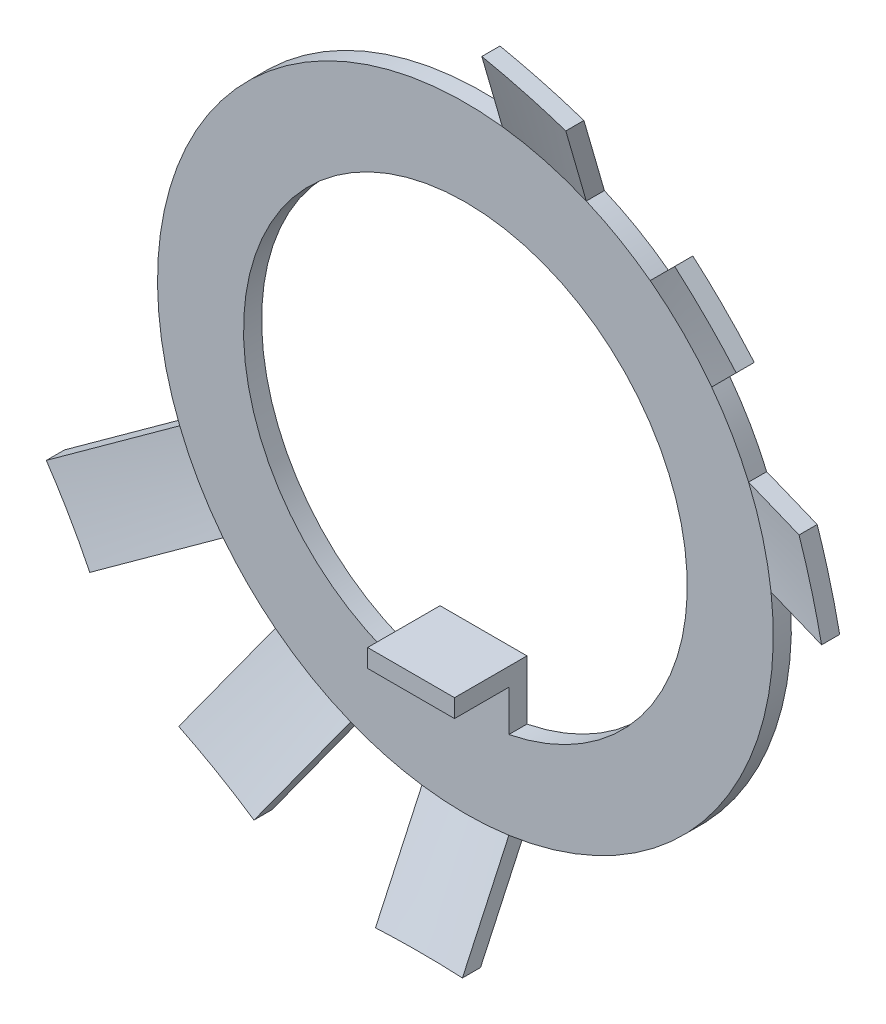
from build123d import *

# Parameters (mm, degrees)
CUT_EXTRUDE2_START  = -3e-06
SKETCH3_OUTSIDE_W   = 59.748
SKETCH3_OUTSIDE_H   = 59.748
CUT_EXTRUDE2_DEPTH  = 3.564697
SKETCH4_W           = 4.8
SKETCH4_H           = 1
BOSS_EXTRUDE1_DEPTH = 4


with BuildPart() as part:
    # Sketch2 → Boss-Revolve (revolve)
    with BuildSketch(Plane(origin=(0, 0, 0), x_dir=(0, 0, -1), z_dir=(1, 0, 0))):
        Polygon((-2.56469212, 22.5), (0, 17), (0, 0), (-1, 0), (-1, 17), (-3.56469212, 22.5), align=None)
    revolve(axis=Axis((0, 0, 0), (0, 0, 1)))

    # Sketch3 outside → Cut-Extrude2 (cut)
    # profile 1 of 2: a face of its own
    with BuildSketch(Plane.XY.offset(CUT_EXTRUDE2_START)):
        Rectangle(SKETCH3_OUTSIDE_W, SKETCH3_OUTSIDE_H)
        with BuildLine():
            Line((-2.4, -16.829735589), (-2.4, -22.371633825))
            Line((-2.4, -22.371633825), (2.4, -22.371633825))
            Line((2.4, -22.371633825), (2.4, -16.829735589))
            ThreePointArc((2.4, -16.829735589), (13.487006785, -10.348944293), (16.877441963, 2.037634111))
            Line((16.877441963, 2.037634111), (22.230504596, 3.471982921))
            Line((22.230504596, 3.471982921), (20.98817318, 8.108426887))
            Line((20.98817318, 8.108426887), (15.635110547, 6.674078078))
            ThreePointArc((15.635110547, 6.674078078), (14.722431864, 8.5), (13.597476435, 10.203363886))
            Line((13.597476435, 10.203363886), (17.516190259, 14.122077709))
            Line((17.516190259, 14.122077709), (14.122077709, 17.516190259))
            Line((14.122077709, 17.516190259), (10.203363886, 13.597476435))
            ThreePointArc((10.203363886, 13.597476435), (8.5, 14.722431864), (6.674078078, 15.635110547))
            Line((6.674078078, 15.635110547), (8.108426887, 20.98817318))
            Line((8.108426887, 20.98817318), (3.471982921, 22.230504596))
            Line((3.471982921, 22.230504596), (2.037634111, 16.877441963))
            ThreePointArc((2.037634111, 16.877441963), (-13.487006785, 10.348944293), (-15.774978559, -6.336406825))
            Line((-15.774978559, -6.336406825), (-20.574403217, -9.107355943))
            Line((-20.574403217, -9.107355943), (-18.174403217, -13.264277882))
            Line((-18.174403217, -13.264277882), (-13.374978559, -10.493328764))
            ThreePointArc((-13.374978559, -10.493328764), (-12.02081528, -12.02081528), (-10.493328764, -13.374978559))
            Line((-10.493328764, -13.374978559), (-13.264277882, -18.174403217))
            Line((-13.264277882, -18.174403217), (-9.107355943, -20.574403217))
            Line((-9.107355943, -20.574403217), (-6.336406825, -15.774978559))
            ThreePointArc((-6.336406825, -15.774978559), (-4.399923767, -16.420739047), (-2.4, -16.829735589))
        make_face(mode=Mode.SUBTRACT)
    # profile 2 of 2: a face of its own
    with BuildSketch(Plane.XY.offset(CUT_EXTRUDE2_START)):
        with BuildLine():
            Line((2.4, -12.012597554), (2.4, -8.75))
            Line((2.4, -8.75), (-2.4, -8.75))
            Line((-2.4, -8.75), (-2.4, -12.012597554))
            ThreePointArc((-2.4, -12.012597554), (0, 12.25), (2.4, -12.012597554))
        make_face()
    extrude(amount=CUT_EXTRUDE2_DEPTH, mode=Mode.SUBTRACT)

    # Sketch4 → Boss-Extrude1 (add)
    with BuildSketch(Plane.XY):
        with Locations((0, -9.25)):
            Rectangle(SKETCH4_W, SKETCH4_H)
    extrude(amount=BOSS_EXTRUDE1_DEPTH)


solid = part.part
